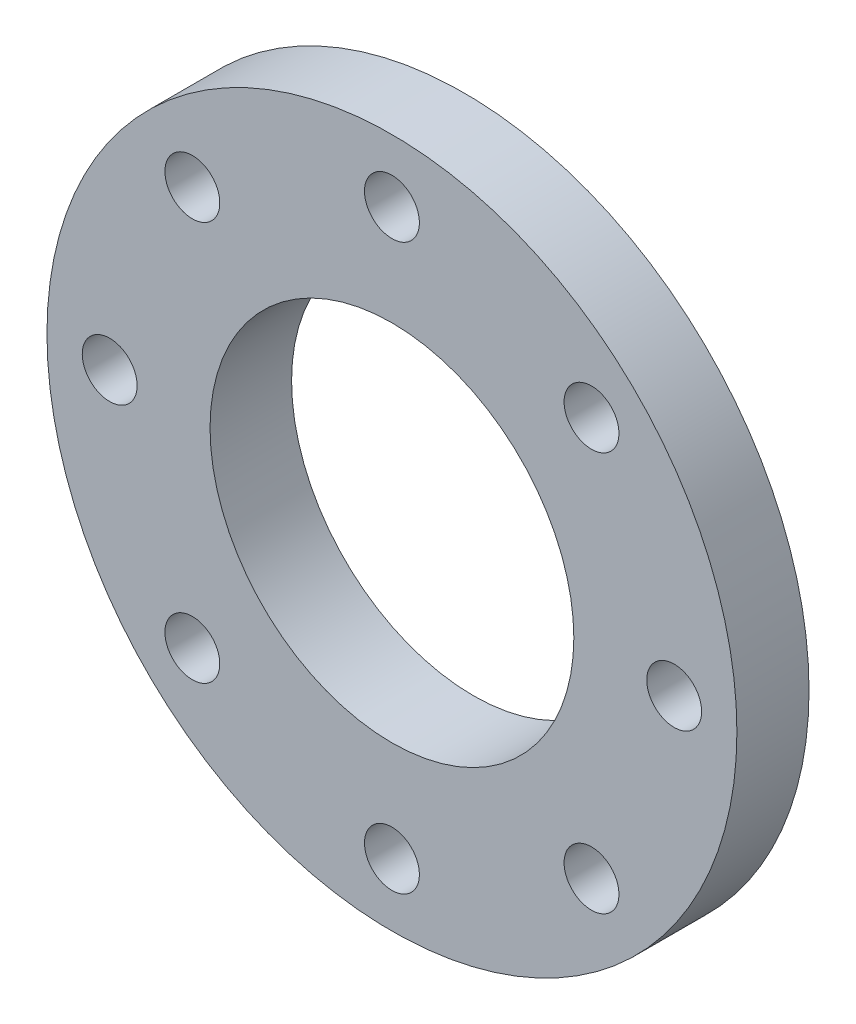
SolidWorks part; units mm, degrees
ref_plane "Front Plane" through (0, 0, 0) normal (0, 0, 1) x (1, 0, 0)
ref_plane "Top Plane" through (0, 0, 0) normal (0, 1, 0) x (1, 0, 0)
ref_plane "Right Plane" through (0, 0, 0) normal (1, 0, 0) x (0, 0, -1)
sketch "Sketch1" plane through (0, 0, 0) normal (0, 0, 1) x (1, 0, 0)
  circle A0 centre (0, 0) radius 110
  circle A1 centre (0, 0) radius 90 construction
  circle A2 centre (0, 90) radius 8.75
  circle A3 centre (63.6396, 63.6396) radius 8.75
  circle A4 centre (90, 0) radius 8.75
  circle A5 centre (63.6396, -63.6396) radius 8.75
  circle A6 centre (0, -90) radius 8.75
  circle A7 centre (-63.6396, -63.6396) radius 8.75
  circle A8 centre (-90, 0) radius 8.75
  circle A9 centre (-63.6396, 63.6396) radius 8.75
  point P22 (0, 0)
  dimension "D1" = 220
  dimension "D2" = 180
  dimension "D3" = 17.5
  dimension "D4" = 8
extrude "Boss-Extrude1" add sketch "Sketch1" along normal blind 26
sketch "Sketch2" plane through (0, 0, 0) normal (0, 0, -1) x (-1, 0, 0)
  circle A0 centre (0, 0) radius 81
  circle A1 centre (0, 0) radius 110
  dimension "D1" = 220
  dimension "D2" = 162
sketch "Sketch3" plane through (0, 0, 0) normal (0, 1, 0) x (1, 0, 0)
  line L0 (0, 0) -> (0, -26) construction
  line L1 (-110, -26) -> (110, -26) construction
  line L3 (-110, 0) -> (-110, -26) construction
  line L4 (-110, -13) -> (110, -13) construction
  line L5 (110, -26) -> (110, 0) construction
  line L6 (110, 0) -> (-110, 0) construction
  line L9 (81, 0) -> (79, 0)
  line L11 (79, 0) -> (81, -3)
  line L12 (81, -3) -> (110, -3)
  line L13 (110, -3) -> (110, 0)
  line L14 (110, 0) -> (81, 0)
  line L15 (81, 0) -> (81, -3) construction
  dimension "D1" = 158
  dimension "D2" = 162
  dimension "D3" = 3
revolve "Cut-Revolve1" cut sketch "Sketch3" angle 360 about L0
sketch "Sketch4" plane through (0, 0, 0) normal (0, 0, -1) x (-1, 0, 0)
  circle A0 centre (0, 0) radius 58
  dimension "D1" = 116
extrude "Cut-Extrude1" cut sketch "Sketch4" against normal through all both and the other way through all
